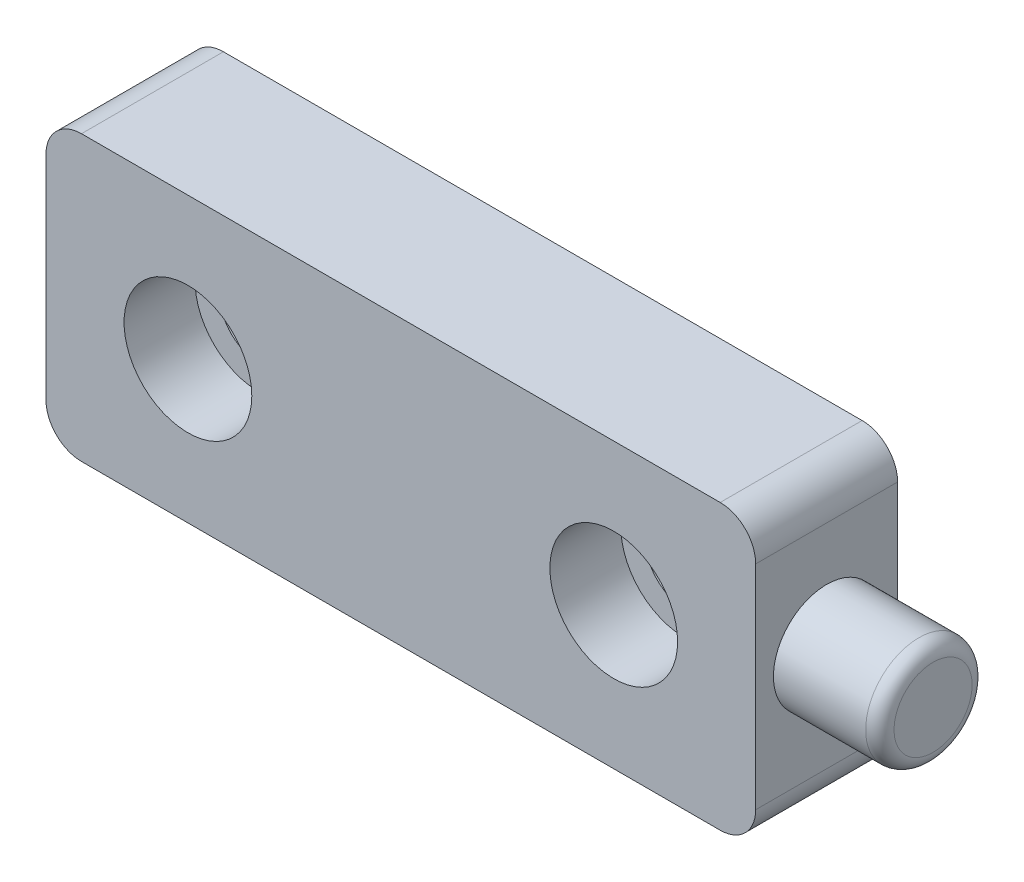
SolidWorks part; units mm, degrees
ref_plane "Front Plane" through (0, 0, 0) normal (0, 0, 1) x (1, 0, 0)
ref_plane "Top Plane" through (0, 0, 0) normal (0, 1, 0) x (1, 0, 0)
ref_plane "Right Plane" through (0, 0, 0) normal (1, 0, 0) x (0, 0, -1)
sketch "Sketch1" plane through (0, 0, 0) normal (0, 0, 1) x (1, 0, 0)
  line L1 (-50, -20) -> (50, -20)
  line L2 (-50, -20) -> (-50, 20)
  line L3 (-50, 20) -> (50, 20)
  line L4 (50, -20) -> (50, 20)
  line L5 (0, 20) -> (0, -20) construction
  line L6 (-50, 0) -> (50, 0) construction
  circle A0 centre (-30, 0) radius 5.5
  circle A1 centre (30, 0) radius 5.5
  point P0 (0, 0)
  dimension "D4" = 11
  dimension "D1" = 40
  dimension "D2" = 100
  dimension "D3" = 60
extrude "Boss-Extrude1" add sketch "Sketch1" along normal mid plane 20
sketch "Sketch2" plane through (50, 0, 0) normal (1, 0, 0) x (0, 0, -1)
  circle A0 centre (0, 0) radius 7.5
  dimension "D1" = 15
extrude "Boss-Extrude2" add sketch "Sketch2" along normal blind 15
fillet "Fillet1" radius 2 1 edges at (65, 0, -7.5)
sketch "Sketch3" plane through (0, 0, 10) normal (0, 0, 1) x (1, 0, 0)
  circle A0 centre (-30, 0) radius 9
  circle A1 centre (30, 0) radius 9
  dimension "D1" = 18
extrude "Cut-Extrude1" cut sketch "Sketch3" against normal blind 10
fillet "Fillet2" radius 5 4 edges at (50, 20, 0) (50, -20, 0) (-50, -20, 0) (-50, 20, 0)
